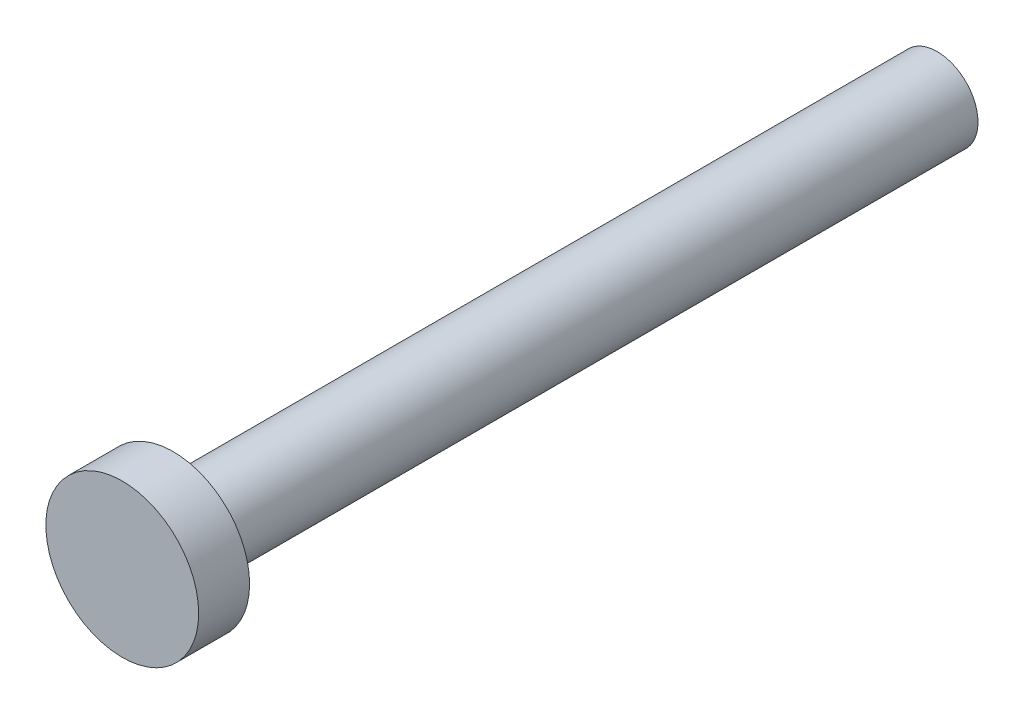
from build123d import *

# Parameters (mm, degrees)
SKETCH1_R           = 4
BOSS_EXTRUDE1_DEPTH = 75
SKETCH2_R           = 7.5
BOSS_EXTRUDE2_DEPTH = 5


with BuildPart() as part:
    # Sketch1 → Boss-Extrude1 (new body)
    with BuildSketch(Plane.XY):
        Circle(SKETCH1_R)
    extrude(amount=BOSS_EXTRUDE1_DEPTH)

    # Sketch2 → Boss-Extrude2 (add)
    with BuildSketch(Plane.XY.offset(75)):
        Circle(SKETCH2_R)
    extrude(amount=BOSS_EXTRUDE2_DEPTH)


solid = part.part
